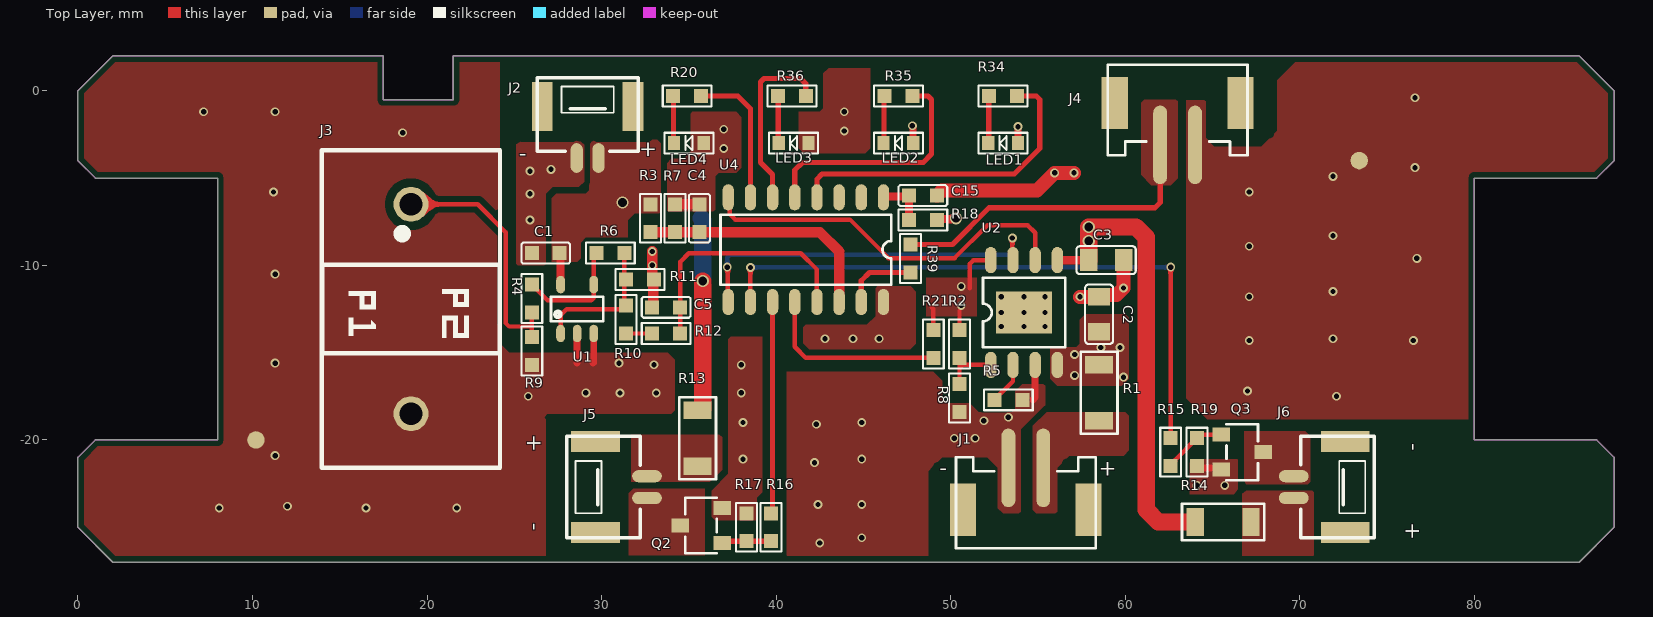
[diagram p0: Top Layer view]
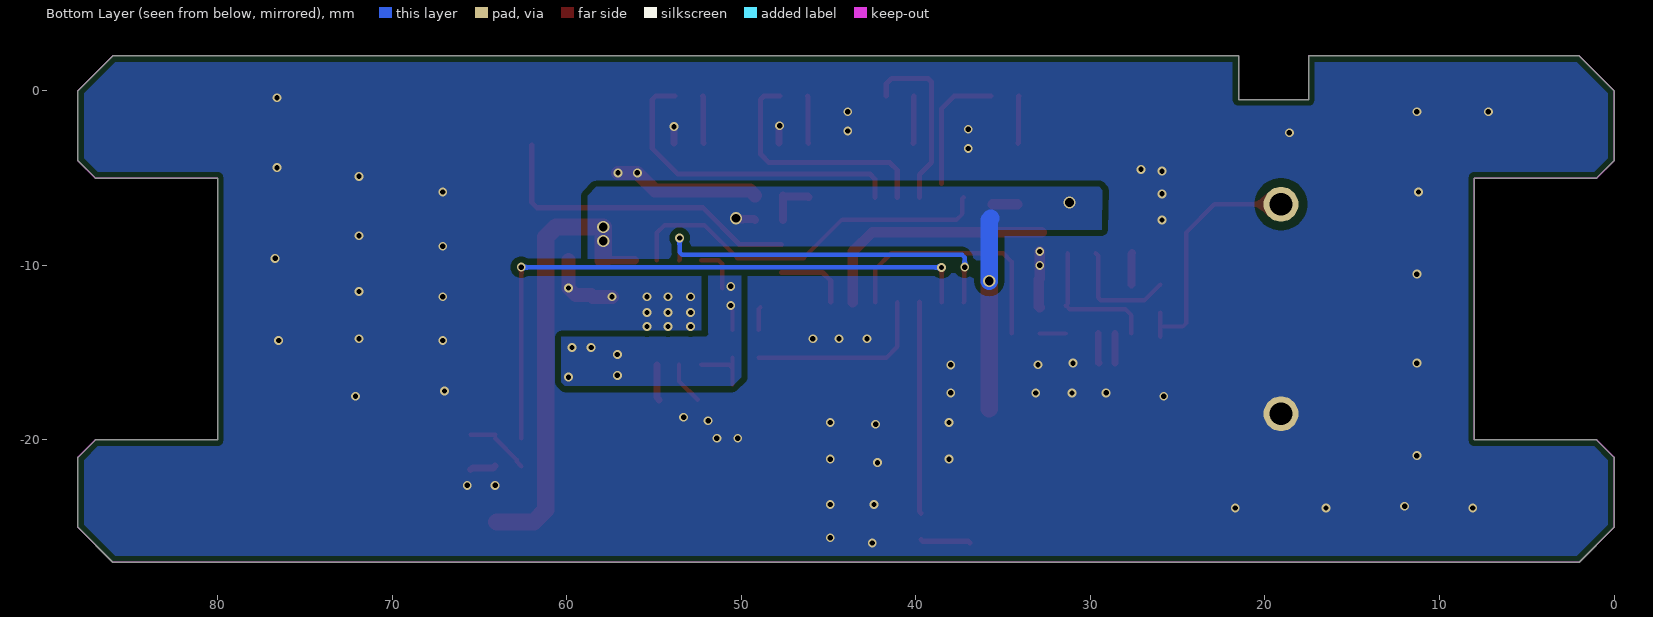
[diagram p1: Bottom Layer view, seen from below]
# Altium PCB MISC75737.PcbDoc
Units mm, origin at the board's own origin, x right, y up, seen from the top; angles counter-clockwise.
Board outline 88 x 29 mm, 2 copper layers (Top Layer, Bottom Layer); 46 components, 36 nets, 130 pads, 93 vias.
Unrouted connection lines stored in the file: 20.

## Layer stack, top to bottom (the 12.6 mil dielectric is the usual default, probably not edited)
Top Solder: solder mask 0.0102, Solder Resist, Dk 3.5
Top Layer: signal copper 0.0356
Dielectric 1: dielectric 0.32, FR-4, Dk 4.8
Bottom Layer: signal copper 0.0356
Bottom Solder: solder mask 0.0102, Solder Resist, Dk 3.5

## Board outline
2,-27 0,-25 0,-21 1,-20 8,-20 8,-5 1,-5 0,-4 0,0 2,2 17.5,2 17.5,-0.5 21.5,-0.5 21.5,2 86,2 88,0 88,-4 87,-5 80,-5 80,-20 87,-20 88,-21 88,-25 86,-27

## Design rules (kind name [scope] priority, off if disabled: settings)
Clearance [All] p1: gap=0.254 ignorepadtopadclearanceinfootprint=FALSE except(0: Arc-Hole Track-Hole SMDPad-Hole THPad-Hole Via-Hole Fill-Hole Poly-Hole Region-Hole Text-Hole; 0.35: Arc-Fill Arc-Poly Arc-Region Track-Fill Track-Poly Track-Region SMDPad-Fill SMDPad-Poly SMDPad-Region THPad-Fill THPad-Poly THPad-Region Via-Fill Via-Poly Via-Region Fill-Fill Fill-Poly Fill-Region Poly-Poly Poly-Region Region-Region)
PolygonConnect [All] p1: connectstyle=Direct reliefconductorwidth=0.254 reliefentries=4 polygonreliefangle="90 Angle" airgapwidth=0.254
RoutingVias [All] p1: holewidth=0.711 width=1.27 viastyle="Through Hole" minholewidth=0.711 minwidth=1.27 maxholewidth=0.711 maxwidth=1.27
SilkToSilkClearance [All] p1: silktosilkclearance=0
SilkToSolderMaskClearance [IsPad] p1: minsilkscreentomaskgap=0 clearancetoexposedcopper=TRUE
SolderMaskExpansion [All] p1: expansion=0.102 istentingtop=FALSE
SupplyNets "Schematic Supply Nets" [InNet('GND')] p1: voltage=0.000
Width [All] p1: maxlimit=1 minlimit=0.254 preferedwidth=0.254
28 further rules are at their usual default settings.

## Components (designator, comment, footprint, x,y, rotation, side; value= is the part's Value field where it differs from the comment)
C1 "100nF/50V" C0603A 26.8,-9.3 r0 top
C2 "10uF/10V" C0805A 58.5,-12.8 r270 top
C3 "10uF/10V" C0805A 58.9,-9.7 r180 top
C4 "100nF/50V" C0603A 35.6,-7.3 r270 top
C5 "NC" C0603A 33.7,-12.4 r0 top
C15 "1uF/10V" C0603A 48.4,-6 r0 top
J1 "Charge" "HY2.0WT-2A/P 立贴带扣耐温260℃" 54.3,-21.6 r0 top
J2 "Battery" GH1.25-2PIN立贴带扣耐温260℃ 29.2,-3.85 r180 top locked
J3 "Current sensor" IND-TH_L18.2-W10.2-P12.00-D0.9_ZHT103 19.08,-12.5 r270 top locked
J4 "Test port" "HY2.0WT-2A/P 立贴带扣耐温260℃" 63,-3.1 r180 top locked
J5 "Blue LED" GH1.25-2PIN立贴带扣耐温260℃ 32.6,-22.7 r270 top locked
J6 "Yellow LED" GH1.25-2PIN立贴带扣耐温260℃ 69.65,-22.7 r90 top locked
LED1 "25%" LED0603A 53,-3 r0 top locked
LED2 "50%" LED0603A 47,-3 r0 top locked
LED3 "75%" LED0603A 41,-3 r0 top locked
LED4 "100%" LED0603A 35,-3 r0 top locked
Q2 "2N7002" SOT23-3L 35.7,-24.9 r90 top
Q3 "2N7002" SOT23-3L 66.7,-20.7 r270 top
R1 "0.5R/1206" R1206A 58.5,-17.3 r90 top
R2 "NC" R0603A 50.5,-14.5 r90 top
R3 "510K/0603 1%" R0603A 32.8,-7.3 r90 top
R4 "1K/0603" R0603A 26,-11.9 r270 top
R5 "1.2K/0603" R0603A 53.3,-17.7 r180 top
R6 "150K/0603" R0603A 30.5,-9.3 r0 top
R7 "200K/0603 1%" R0603A 34.2,-7.3 r270 top
R8 "NC" R0603A 50.5,-17.6 r90 top
R9 "2K/0603" R0603A 26,-14.9 r270 top
R10 "1K/0603" R0603A 31.4,-13.1 r270 top
R11 "10K/0603" R0603A 32.2,-10.8 r0 top
R12 "0R/0603" R0603A 33.7,-13.9 r0 top
R13 "10R/1206" R1206A 35.5,-19.9 r270 top
R14 "10R/1206" R1206A 65.6,-24.7 r0 top
R15 "1K" R0603A 62.6,-20.7 r90 top
R16 "1K" R0603A 39.7,-25 r90 top
R17 "100K" R0603A 38.3,-25 r270 top
R18 "1R" R0603A 48.4,-7.4 r180 top
R19 "100K" R0603A 64.1,-20.7 r90 top
R20 "100R/5%" R0603A 34.9,-0.3 r0 top
R21 "NC" R0603A 49,-14.5 r90 top
R34 "100R/5%" R0603A 53,-0.3 r0 top
R35 "100R/5%" R0603A 47,-0.3 r0 top
R36 "100R/5%" R0603A 40.9,-0.3 r0 top
R39 "1K" R0603A 47.7,-9.6 r90 top
U1 "LM321" SOT23-5A 28.6,-12.5 r90 top
U2 "4056" ESOP-8L 54.2,-12.7 r90 top
U4 "ZM072" SOP16L 41.7,-9.1 r270 top

## Footprints (in the part's own frame and the unit in brackets; to place one, negate y for a bottom-side part, rotate by r counter-clockwise, add the part's x,y. Pads: shape width x height; smd on the part's side, far side on the other; paste and mask are expansions set on the pad)
C0603A [mm] "贴片电容"
  rect 0.8x0.8 smd mask+0.08: 1(-0.8,0) 2(0.8,0)
  silkscreen extent -1.4,-0.6 1.4,0.6
C0805A [mm] "贴片电容"
  rect 1x1.25 smd: 1(-1,0)
  rect 1x1.25 smd mask+0.102: 2(1,0)
  silkscreen extent -1.7,-0.8 1.7,0.8
ESOP-8L [mm] "贴片MOS/IC"
  rect 2.4x3.2 smd: 0(0,0)
  oval 1.5x0.65 smd: 1(-3,1.905) 2(-3,0.635) 3(-3,-0.635) 4(-3,-1.905) 5(3,-1.905) 6(3,-0.635) 7(3,0.635) 8(3,1.905)
  silkscreen extent -2,-2.35 2,2.35
GH1.25-2PIN立贴带扣耐温260℃ [mm] "立贴带扣耐温260℃"
  rect 1.2x2.8 smd: 0(-2.6,-2.95) 0(2.6,-2.95)
  oval 0.7x1.7 smd: 1(-0.625,0) 2(0.625,0)
  silkscreen extent -2.9,-4.6 2.9,-0.4
"HY2.0WT-2A/P 立贴带扣耐温260℃" [mm] "卧贴连接器"
  rect 1.5x3 smd: 0(-3.6,-2.4) 0(3.6,-2.4)
  oval 0.8x4.5 smd: 1(-1,0) 2(1,0)
  silkscreen extent -4,-4.6 4,0.6
IND-TH_L18.2-W10.2-P12.00-D0.9_ZHT103 [mm]
  round 2 hole 1.3: 1(-6,0) 2(6,0)
  silkscreen extent -9.1,-5.1 9.1,5.1
LED0603A [mm] "贴片LED"
  rect 0.7x0.8 smd: 1(-0.85,0) 2(0.85,0)
  silkscreen extent -1.4,-0.6 1.4,0.6
R0603A [mm] "贴片电阻"
  rect 0.8x0.8 smd mask+0.08: 1(-0.8,0) 2(0.8,0)
  silkscreen extent -1.4,-0.6 1.4,0.6
R1206A [mm] "贴片电阻"
  rect 1x1.6 smd: 1(-1.6,0) 2(1.6,0)
  silkscreen extent -2.35,-1.05 2.35,1.05
SOP16L [mm]
  oval 1.5x0.65 smd: 1(-3,4.445) 2(-3,3.175) 3(-3,1.905) 4(-3,0.635) 5(-3,-0.635) 6(-3,-1.905) 7(-3,-3.175) 8(-3,-4.445) 9(3,-4.445) 10(3,-3.175) 11(3,-1.905) 12(3,-0.635) 13(3,0.635) 14(3,1.905) 15(3,3.175) 16(3,4.445)
  silkscreen extent -2,-4.89 2,4.89
SOT23-3L [mm] "贴片IMOS"
  rect 0.8x1 smd: 1(-1,-1.2) 2(1,-1.2) 3(0,1.2)
  silkscreen extent -1.6,-0.9 1.6,0.9
SOT23-5A [mm] "贴片IC"
  oval 1x0.5 smd mask+0.05: 1(-1.4,0.95) 2(-1.4,0) 3(-1.4,-0.95) 4(1.4,-0.95) 5(1.4,0.95)
  silkscreen extent -0.7,-1.5 0.7,1.5

## Part data
C1 C4 C5: library part Cap0603
C2 C3: library part Cap0805, "SMD capacitor"
C15: library part CH
J1 J2 J3 J4 J5 J6: library part 2PIN, "DC socket right-angle 90° pitch 2.0"
LED1 LED2 LED3 LED4: library part "LED 白发蓝", "SMD LED"
Q2 Q3: "SMD MOS"
R1 R13 R14: library part Res1206, "SMD resistor"
R2 R3 R4 R5 R6 R7 R8 R9 R10 R11 R12 R15 R16 R17 R19 R20 R21 R34 R35 R36 R39: library part Res0603, "SMD resistor"
R18: library part RH1
U2: library part TP4056, "Charger IC"
U4: library part MCU-TSSOP-16

## Free pads (board coordinates)
  round 1 smd: 2(10.2,-20) 3(73.4,-4)

## Via types
v1: diameter 0.508, hole 0.305, Top Layer to Bottom Layer, tented both sides, 88 vias
v2: diameter 0.7, hole 0.5, Top Layer to Bottom Layer, tented both sides, 5 vias

## Nets (pads, with @x,y where several pads share a name; then routed paths per layer and width w, separated by ;. In a path a pad name is that pad's centre, name@x,y a point inside that pad or via, vN(x,y) a via of type N, cw(c..) or ccw(c..) an arc to the next point about the centre after c; other vN are vias at no path point)
BAT+: C1.2 C3.2 J2.1 R3.2 R13.1 R14.1 R18.1 U1.5 U2.5 | length 40
  Top Layer w0.45: C1.2 27.64,-9.34 27.64,-11.09 U1.5 ; R18.1 49.252,-7.348 50.252,-7.348 v2(50.3,-7.3)
  Top Layer w0.5: U2.5 C3.2 C3.2@58.1,-9.7
  Top Layer w1: R13.1@35.8,-18.2 v2(35.8,-10.9) ; C3.2 v2(57.9,-8.6) v2(57.9,-7.8) 60.6,-7.8 61.2,-8.4 61.2,-24 61.9,-24.7 R14.1
  Bottom Layer w1: 35.7,-7.3 35.8,-7.4 v2(35.8,-10.9)
  other v2: 31.2,-6.4
CURR: C5.2 R12.2 U4.13 | length 14.4
  Top Layer w0.254: R12.2 C5.2 34.5,-9.8 35,-9.3 41.4,-9.3 42.335,-10.235 U4.13
EN: C2.2 R1.2 R2.2 R21.2 U2.4 U2.8 | length 5.1
  Top Layer w0.254: 48.9,-12.4 49,-12.5 R21.2 ; R2.2 50.5,-12.6 ; 51.1,-11.3 51.1,-9.9 51.3,-9.7 U2.8
  other v1: 59.9,-16.4 57.1,-16.3 57.1,-15.1 58.6,-14.7 59.7,-14.7 50.6,-12.3 50.6,-11.2
FULL: U2.6 U4.8 | length 22.1
  Top Layer w0.254: U4.8 37.331,-6.176 37.331,-7.051 37.655,-7.376 44.226,-7.376 46.432,-9.581 50.219,-9.581 52.1,-7.7 54.4,-7.7 54.835,-8.135 U2.6
GHG: U2.7 U4.9 | length 21.1
  Top Layer w0.254: v1(37.2,-10.1) 37.228,-10.128 37.228,-12.072 U4.9 ; v1(53.532,-8.432) 53.532,-9.667 U2.7
  Bottom Layer w0.254: v1(37.2,-10.1) 37.2,-9.549 37.349,-9.4 53.384,-9.4 53.532,-9.251 v1(53.532,-8.432)
GND: C1.1 C2.1 C3.1 C4.1 C5.1 C15.2 J1.1 J2.2 J3.2 J4.1 LED1.2 LED2.2 LED3.2 LED4.2 pad.2 pad.3 Q2.2 Q3.2 R5.1 R7.1 R8.1 R9.2 R11.2 R17.1 R19.1 U1.2 U1.3 U2.0 U2.3 U4.16 | length 26.3
  Top Layer w0.4: 28.6,-15.6 U1.2 ; 29.5,-15.6 29.55,-15.55 U1.3 ; v1(47.8,-2) 47.8,-2.029 47.85,-2.079 LED2.2 ; LED1.2 v1(53.85,-2.05) ; 54.7,-17.7 54.835,-17.565 U2.3 ; R19.1 64.2,-21.6 65.4,-21.6 Q3.2
  Top Layer w0.6: C5.1 32.95,-12.35 32.95,-10.8 32.9,-10.75 v1(32.9,-9.2) ; R7.1 C4.1
  Top Layer w0.8: C15.2 49.5,-5.7 54.951,-5.7 v1(55.951,-4.7) v1(57.065,-4.7) ; v1(57.4,-11.8) C2.1 58.6,-11.7 59.5,-11.7 v1(59.9,-11.3) C3.1
  other v1: 42.5,-25.9 44.9,-25.6 8.1,-23.9 16.5,-23.9 21.7,-23.9 12,-23.8 42.4,-23.7 44.9,-23.7 64.1,-22.6 65.7,-22.6 42.2,-21.3 38.1,-21.1 44.9,-21.1 11.3,-20.9 50.2,-19.9 51.4,-19.9 42.3,-19.1 38.1,-19 44.9,-19 51.9,-18.9 53.3,-18.7 25.8,-17.5 72.1,-17.5 31.057,-17.315 33.133,-17.315 29.1,-17.3 38,-17.3 67,-17.2 33.006,-15.694 38,-15.7 11.3,-15.6 31,-15.6 67.1,-14.3 76.5,-14.3 42.8,-14.2 44.4,-14.2 45.9,-14.2 71.9,-14.2 52.9,-13.5 54.2,-13.5 55.4,-13.5 52.9,-12.7 54.2,-12.7 55.4,-12.7 52.9,-11.8 54.2,-11.8 55.4,-11.8 67.1,-11.8 71.9,-11.5 11.3,-10.5 32.9,-10 76.7,-9.6 67.1,-8.9 71.9,-8.3 25.9,-7.4 25.9,-5.9 11.2,-5.8 67.1,-5.8 71.9,-4.9 25.9,-4.6 27.1,-4.5 76.6,-4.4 37,-3.3 18.6,-2.4 43.9,-2.3 37,-2.2 7.2,-1.2 11.3,-1.2 43.9,-1.2 76.6,-0.4
ICPCL: U4.3
ICPDA: U4.2
LED1: LED1.1 R34.1 | length 2.7
  Top Layer w0.3: LED1.1 52.175,-2.975 52.175,-0.325 R34.1
LED2: LED2.1 R35.1 | length 2.7
  Top Layer w0.3: LED2.1 46.175,-2.975 46.175,-0.325 R35.1
LED3: LED3.1 R36.1 | length 2.7
  Top Layer w0.3: R36.1 40.125,-0.325 40.125,-2.975 LED3.1
LEDB: R16.2 U4.11 | length 12.1
  Top Layer w0.3: R16.2 39.795,-24.105 U4.11
LEDY: R15.2 U4.10 | length 35.9
  Top Layer w0.254: U4.10 v1(38.525,-10.125) ; R15.2 v1(62.6,-10.1)
  Bottom Layer w0.254: v1(38.525,-10.125) 38.538,-10.112 62.587,-10.112 v1(62.6,-10.1)
NetC15_1: C15.1 R18.2 U4.1 | length 2.9
  Top Layer w0.45: U4.1 46.195,-6.05 47.55,-6.05 C15.1 R18.2
NetJ1_2: J1.2 R1.1
NetJ3_1: J3.1 R4.2 R9.1 | length 14.3
  Top Layer w0.254: J3.1 22.9,-6.5 24.5,-8.1 24.5,-13.3 24.7,-13.5 26,-13.5 ; R9.1 26,-13.5 ; R4.2 26,-13.5
NetJ4_2: J4.2 R39.2 | length 18.6
  Top Layer w0.3: R39.2 50.1,-8.8 52.2,-6.7 61.7,-6.7 62,-6.4 J4.2
NetJ5_1: J5.1 R13.2
NetJ5_2: J5.2 Q2.3
NetJ6_1: J6.1 R14.2
NetJ6_2: J6.2 Q3.3
NetLED4_1: LED4.1 R20.1 | length 2.7
  Top Layer w0.3: R20.1 34.125,-0.325 34.125,-2.975 LED4.1
NetQ2_1: Q2.1 R16.1 R17.2 | length 2.9
  Top Layer w0.3: Q2.1 37,-25.8 R17.2 39.6,-25.8 R16.1@39.7,-25.7
NetQ3_1: Q3.1 R15.1 R19.2 | length 3.6
  Top Layer w0.254: R15.1 62.873,-21.227 62.873,-21.127 R19.2 ; R19.2@64.1,-19.7 Q3.1
NetR2_1: R2.1 R8.2 U2.1 | length 3.4
  Top Layer w0.254: R8.2 50.5,-15.9 ; R2.1 50.5,-15.9 ; U2.1 50.7,-15.7 50.5,-15.9
NetR4_1: R4.1 R6.1 U1.4 | length 6.6
  Top Layer w0.254: R4.1 26.9,-12 29.401,-12 29.55,-11.851 29.55,-9.45 R6.1
NetR5_2: R5.2 U2.2 | length 2.4
  Top Layer w0.254: R5.2 53.565,-16.635 U2.2
NetR6_2: R6.2 R10.1 R11.1 U1.1 | length 8.1
  Top Layer w0.254: U1.1 27.65,-12.85 27.992,-12.508 31.192,-12.508 R10.1 31.3,-12.2 R6.2
NetR10_2: R10.2 R12.1 | length 1.5
  Top Layer w0.254: R10.2 R12.1
NetR20_2: R20.2 U4.7 | length 7.4
  Top Layer w0.3: R20.2 37.8,-0.3 38.525,-1.025 38.525,-5.3
NetR21_1: R21.1 U4.12 | length 10.8
  Top Layer w0.254: U4.12 41.065,-14.665 41.7,-15.3 R21.1
NetR34_2: R34.2 U4.4 | length 18.7
  Top Layer w0.3: U4.4 42.335,-5.065 42.635,-4.765 53.635,-4.765 55.1,-3.3 55.1,-0.5 54.9,-0.3 R34.2
NetR35_2: R35.2 U4.5 | length 14.1
  Top Layer w0.3: U4.5 41.065,-4.535 41.5,-4.1 48.424,-4.1 48.9,-3.624 48.9,-0.5 48.7,-0.3 R35.2
NetR36_2: R36.2 U4.6 | length 10.4
  Top Layer w0.3: U4.6 39.795,-4.795 39.1,-4.1 39.1,0.5 39.3,0.7 41.4,0.7 41.7,0.4 R36.2
NetR39_1: R39.1 U4.15 | length 4.2
  Top Layer w0.3: U4.15 44.875,-10.876 45.351,-10.4 R39.1
VBAT1: C4.2 R3.1 R7.2 U4.14 | length 14.2
  Top Layer w0.6: R3.1 R7.2 C4.2 42.5,-8.1 43.605,-9.205 U4.14
pads on no net: J1.0 J2.0 J4.0 J5.0 J6.0

## Polygon pours and split planes (outlines as drawn)
GND on Top Layer "NONET_L02_P-001" (solid, remove dead copper, pour order 18): 63.5,-0.529 64.529,-0.529 64.6,-0.6 64.6,-2.7 65.1,-3.2 67.8,-3.2 68.7,-2.3 68.7,0.6 70.1,2 88.3,2 88.5,1.8 88.5,-18.3 88,-18.8 64.7,-18.8 63.5,-17.6
GND on Top Layer "NONET_L02_P-001" (solid, remove dead copper, pour order 12): 49,-16.1 49.5,-16.6 49.5,-17.6 49.8,-17.9 51.1,-17.9 51.6,-18.4 53.5,-18.4 53.7,-18.2 53.7,-17.2 54.1,-16.8 55.3,-16.8 55.4,-16.9 55.4,-18 54,-19.4 54,-21.4 54,-22.5 54,-24.1 53.9,-24.2 53,-24.2 52.7,-23.9 52.7,-21.6 52.1,-21 49.5,-21 48.7,-21.8 48.7,-27 41,-27 40.6,-26.6 40.6,-16.1
NetJ1_2 on Top Layer "NONET_L02_P-001" (solid, remove dead copper, pour order 11): 60,-18.4 60.2,-18.6 60.2,-19.4 60.2,-20.6 59.9,-20.9 56.8,-20.9 56.1,-21.6 56.1,-24.1 56,-24.2 54.9,-24.2 54.7,-24 54.7,-19.2 55.5,-18.4
GND on Top Layer "NONET_L02_P-001" (solid, remove dead copper, pour order 0): 26.9,-18.5 26.7,-18.7 26.8,-18.8 26.8,-26.8 26,-27.6 2,-27.6 -1.3,-24.3 -1.3,3.9 23.1,3.6 24.16,2.54 24.16,-14.46 24.7,-15 33.8,-15 34.2,-15.4 34.2,-18.3 34,-18.5
NetJ4_2 on Top Layer "NONET_L02_P-001" (solid, remove dead copper, pour order 23): 61.071,-0.5 60.9,-0.671 60.9,-4.8 61.5,-5.4 62.6,-5.4 63,-5 63,-0.6 62.9,-0.5
GND on Top Layer "NONET_L02_P-001" (solid, remove dead copper, pour order 20): 66.443,-21.143 66.443,-22.857 66.2,-23.1 63.7,-23.1 63.7,-21.3 63.9,-21.1 66.4,-21.1
GND on Top Layer "NONET_L02_P-001" (solid, remove dead copper, pour order 19): 45.7,-11.3 45.7,-12.9 45.2,-13.4 43.65,-13.4 41.7,-13.4 41.5,-13.6 41.5,-14.5 41.9,-14.9 47.6,-14.9 48,-14.5 48,-11.5 47.7,-11.2 45.8,-11.2
GND on Top Layer "NONET_L02_P-001" (solid, remove dead copper, pour order 16): 41.3,-1.2 41.3,-3.3 41.6,-3.6 45.1,-3.6 45.4,-3.3 45.4,1.3 43,1.3 42.7,1 42.7,-1 42.5,-1.2 41.4,-1.2
EN on Top Layer "NONET_L02_P-001" (solid, remove dead copper, pour order 14): 48.6,-10.7 48.6,-12.9 51.5,-12.9 51.5,-10.7
EN on Top Layer "NONET_L02_P-001" (solid, remove dead copper, pour order 10): 55.7,-14.7 55.7,-16.5 56.1,-16.9 59.8,-16.9 60.2,-16.5 60.2,-13 60,-12.8 57.7,-12.8 57.4,-13.1 57.4,-14.5 57.2,-14.7
NetJ6_2 on Top Layer "NONET_L02_P-001" (solid, remove dead copper, pour order 9): 66.8,-19.5 70.3,-19.5 70.6,-19.8 70.6,-22.4 70.4,-22.6 66.8,-22.6
NetJ6_1 on Top Layer "NONET_L02_P-001" (solid, remove dead copper, pour order 8): 70.8,-26.6 70.8,-23 70.7,-22.9 66.933,-22.9 66.7,-23.075 66.7,-26.7 66.9,-26.9 70.5,-26.9
GND on Top Layer "NONET_L02_P-001" (solid, remove dead copper, pour order 6): 35.1,-3.5 34.7,-3.9 34,-3.9 33.7,-4.2 33.7,-6.8 33.812,-6.912 36.388,-6.912 36.5,-6.8 36.5,-4.9 36.7,-4.7 37.7,-4.7 38,-4.4 38,-1.5 37.7,-1.2 35.2,-1.2 35.1,-1.3
GND on Top Layer "NONET_L02_P-001" (solid, remove dead copper, pour order 5): 39.2,-23 38.9,-23.3 38.9,-24.6 36.5,-24.6 36.3,-24.4 36.3,-22.9 37.257,-21.943 37.257,-14.243 37.4,-14.1 39.2,-14.1
NetJ5_1 on Top Layer "NONET_L02_P-001" (solid, remove dead copper, pour order 4): 31.7,-22.4 36.2,-22.4 36.5,-22.1 36.9,-21.7 36.9,-19.85 36.75,-19.7 31.7,-19.7
NetJ5_2 on Top Layer "NONET_L02_P-001" (solid, remove dead copper, pour order 3): 31.55,-26.6 31.55,-23.05 31.8,-22.8 35.9,-22.8 35.9,-26.6
BAT+ on Top Layer "NONET_L02_P-001" (solid, remove dead copper, pour order 2): 27.1,-9.8 28.6,-9.8 28.8,-9.6 28.8,-8.7 29.1,-8.4 31.5,-8.4 31.5,-7.4 31.9,-7 33.3,-7 33.4,-6.9 33.4,-3 33.2,-2.8 29.4,-2.8 29.3,-2.9 29.3,-5.7 29.1,-5.9 27.4,-5.9 27.1,-6.2
GND on Top Layer "NONET_L02_P-001" (solid, remove dead copper, pour order 1): 28.25,-5.5 28.7,-5.5 29,-5.2 29,-3.1 28.7,-2.8 25.2,-2.8 25.1,-2.9 25.1,-9.9 25.2,-10 26.7,-10 26.8,-9.9 26.8,-5.9 27.2,-5.5
GND on Bottom Layer "GND_L02_P015" (solid, remove dead copper, pour order 15): 2,-27 0,-25 0,-21 1,-20 8,-20 8,-5 1,-5 0,-4 0,0 2,2 17.5,2 17.5,-0.5 21.5,-0.5 21.5,2 86,2 88,0 88,-4 87,-5 80,-5 80,-20 87,-20 88,-21 88,-25 86,-27
EN on Bottom Layer "NONET_L02_P-001" (solid, remove dead copper, pour order 13): 50.5,-16.9 50,-16.4 50,-12.9 50,-10.6 50.1,-10.5 51.9,-10.5 51.9,-13.9 51.85,-13.95 52,-14.1 60.3,-14.1 60.3,-16.7 60.1,-16.9
BAT+ on Bottom Layer "NONET_L02_P-001" (solid, remove dead copper, pour order 7): 35.3,-8 35.25,-7.95 29.359,-7.95 29.309,-5.5 58.3,-5.5 58.8,-6 58.8,-9.7 35.7,-9.7 35.3,-9.3

## Keep-outs
Keep-Out Layer:
  the board outline again, w0.013

## Other copper
Top Layer:
  pour cut-out: 19.08,-8 cw(c19.08,-6.5) 17.58,-6.5 cw(c19.08,-6.5) 19.08,-5 cw(c19.08,-6.5) 20.58,-6.5 cw(c19.08,-6.5)
Bottom Layer:
  pour cut-out: 19.08,-8 cw(c19.08,-6.5) 17.58,-6.5 cw(c19.08,-6.5) 19.08,-5 cw(c19.08,-6.5) 20.58,-6.5 cw(c19.08,-6.5)

## Silkscreen, mask and mechanical layers (free items; w line width, h text height)
Top Overlay:
  text "+" at 33.2,-2.659 h1.52 r180
  text "-" at 25.7,-3.039 h1.52 r180
  text "-" at 75.839,-20.2 h1.52 r270
  text "+" at 26.841,-20.7 h1.52 r90
  text "+" at 59.5,-20.959 h1.52 r180
  text "-" at 49.8,-21.039 h1.52 r180
  text "+" at 75.759,-24.7 h1.52 r270
  text "-" at 26.761,-25.2 h1.52 r90